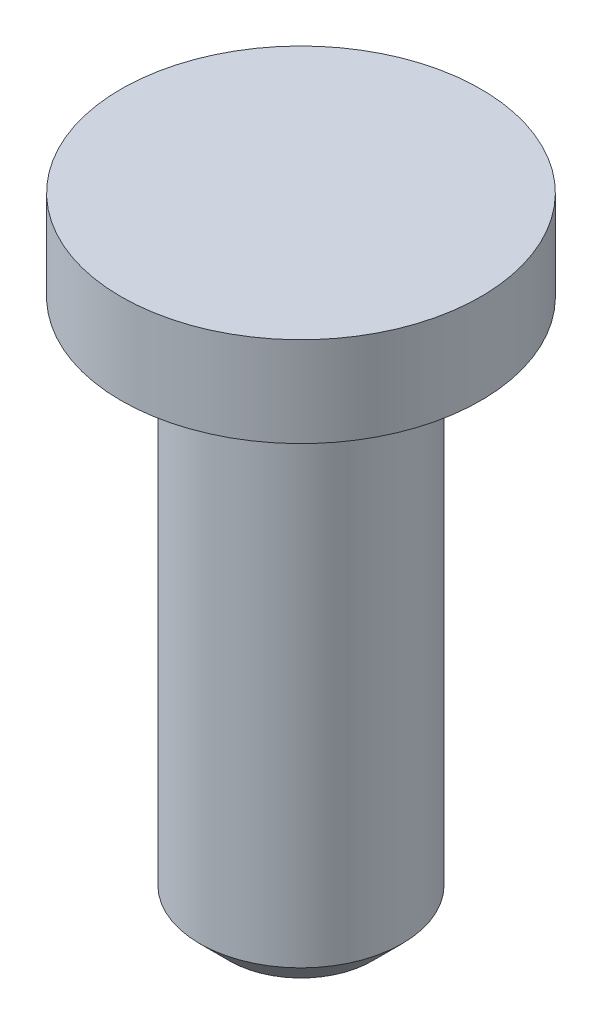
from build123d import *

# Parameters (mm, degrees)
CHAMFER1_SIZE = 1


with BuildPart() as part:
    # Sketch1 → Revolve2 (revolve)
    with BuildSketch(Plane.XY, mode=Mode.PRIVATE) as revolve2_sk:
        Polygon((-158.944232661, -426.85207641), (-162.319232661, -426.85207641), (-162.319232661, -405.85207641), (-156.319232661, -405.85207641), (-156.319232661, -408.85207641), (-158.944232661, -408.85207641), align=None)
    revolve(revolve2_sk.sketch.rotate(Axis((-162.319232661, -405.85207641, 0), (0, -1, 0)), 90), axis=Axis((-162.319232661, -405.85207641, 0), (0, -1, 0)))

    # Chamfer1
    chamfer1_edges = [part.edges().sort_by_distance(p)[0] for p in [
        (-162.319232661, -426.85207641, -3.375),
    ]]
    chamfer(chamfer1_edges, length=CHAMFER1_SIZE)


solid = part.part
